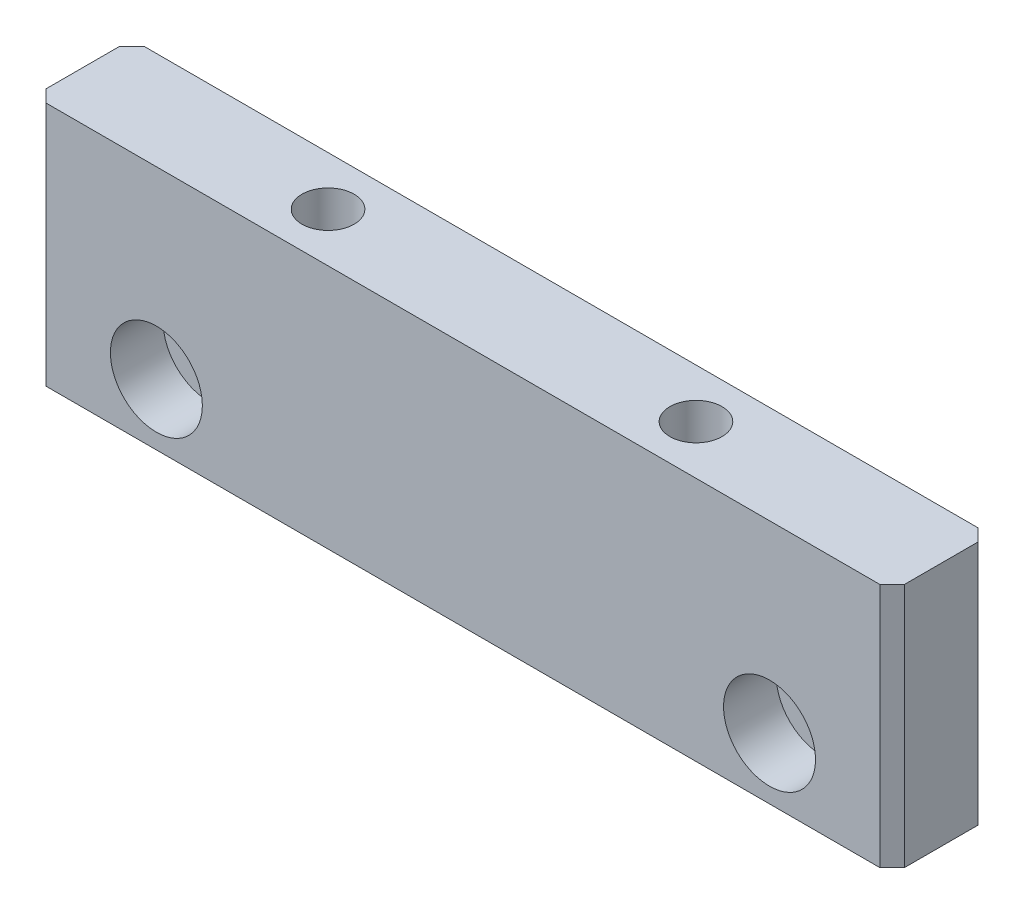
from build123d import *

# Parameters (mm, degrees)
SKETCH_1_W                   = 140
SKETCH_1_H                   = 40
EXTRUDE_1_DEPTH              = 16
HOLE_WIZARD_M10_1_D          = 8.5
HOLE_WIZARD_M8_1_D           = 8.4
HOLE_WIZARD_M8_1_CBORE_D     = 15
HOLE_WIZARD_M8_1_CBORE_DEPTH = 8.6
CHAMFER_1_SIZE               = 2


with BuildPart() as part:
    # 草图1 → 凸台-拉伸1 (new body)
    with BuildSketch(Plane.XY):
        with Locations((70, 20)):
            Rectangle(SKETCH_1_W, SKETCH_1_H)
    extrude(amount=EXTRUDE_1_DEPTH)

    # M10 螺纹孔1 (through all)
    with Locations(Plane(origin=(0, 40, 0), x_dir=(1, 0, 0), z_dir=(0, 1, 0))):
        with Locations((40, -8), (100, -8)):
            Hole(HOLE_WIZARD_M10_1_D / 2)

    # M8 六角凹头螺钉的柱形沉头孔1 (through all)
    with Locations(Plane.XY.offset(16)):
        with Locations((20, 10), (120, 10)):
            CounterBoreHole(HOLE_WIZARD_M8_1_D / 2, HOLE_WIZARD_M8_1_CBORE_D / 2, HOLE_WIZARD_M8_1_CBORE_DEPTH)

    # 倒角1
    chamfer_1_edges = [part.edges().sort_by_distance(p)[0] for p in [
        (140, 20, 16),
        (0, 20, 16),
        (140, 20, 0),
        (0, 20, 0),
    ]]
    chamfer(chamfer_1_edges, length=CHAMFER_1_SIZE)


solid = part.part
